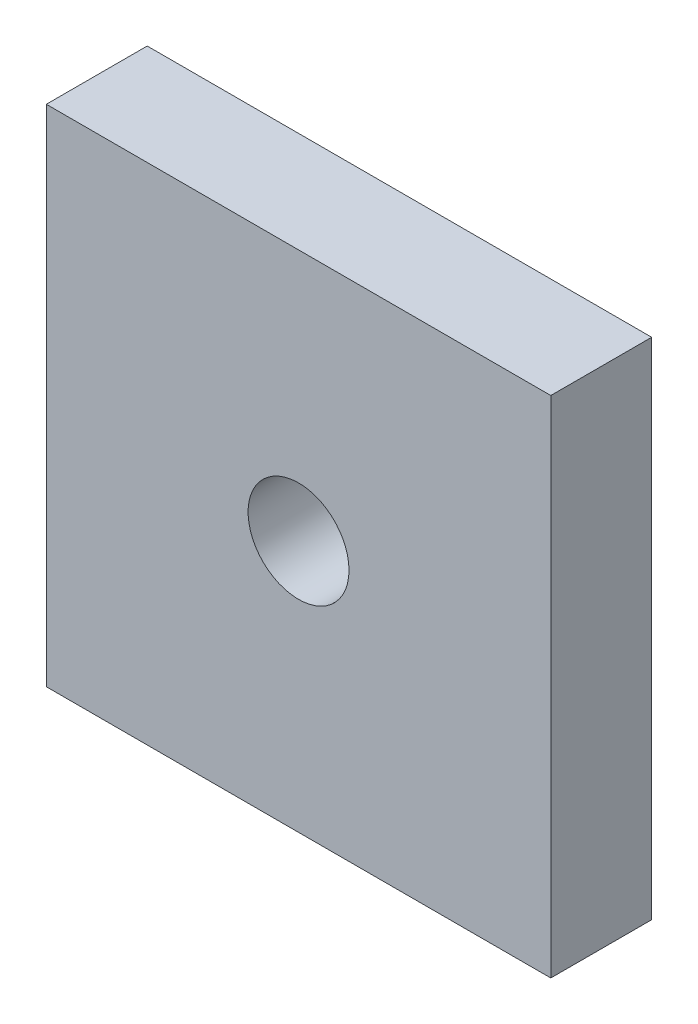
from build123d import *

# Parameters (mm, degrees)
SKETCH_1_W      = 50
SKETCH_1_H      = 50
SKETCH_1_R      = 5
EXTRUDE_1_DEPTH = 10


with BuildPart() as part:
    # 草图1 → 凸台-拉伸1 (new body)
    with BuildSketch(Plane.XY):
        with Locations((25, 25)):
            Rectangle(SKETCH_1_W, SKETCH_1_H)
        with Locations((25, 25)):
            Circle(SKETCH_1_R, mode=Mode.SUBTRACT)
    extrude(amount=EXTRUDE_1_DEPTH)


solid = part.part
